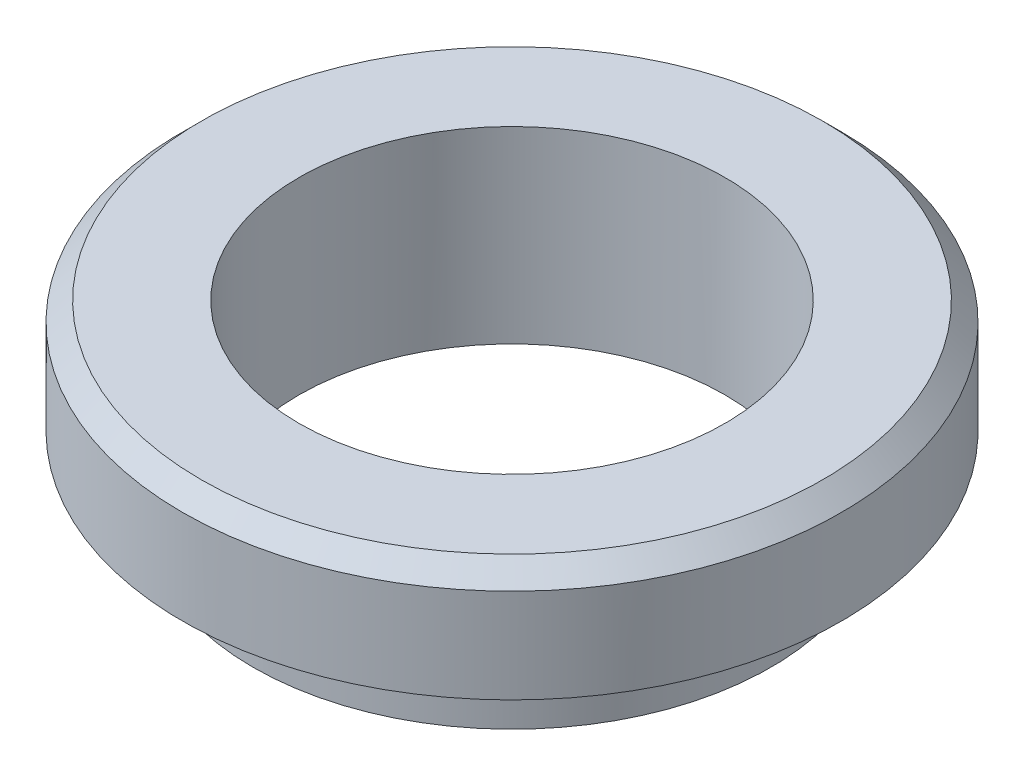
from build123d import *

# Parameters (mm, degrees)
G1_1_2_TAPPED_HOLE1_D     = 45.25
G1_1_2_TAPPED_HOLE1_DEPTH = 102.54
G1_1_2_TAPPED_HOLE1_TIP   = 13.594471505
CHAMFER1_SIZE             = 2


with BuildPart() as part:
    # Sketch1 → Revolve1 (revolve)
    with BuildSketch(Plane.XY, mode=Mode.PRIVATE) as revolve1_sk:
        Polygon((0, 0), (35, 0), (35, -12), (27.5, -12), (27.5, -20), (0, -20), align=None)
    revolve(revolve1_sk.sketch.rotate(Axis((0, -20, 0), (0, 1, 0)), 90), axis=Axis((0, -20, 0), (0, 1, 0)))

    # G1-1/2 Tapped Hole1
    with Locations(Plane(origin=(0, 0, 0), x_dir=(1, 0, 0), z_dir=(0, 1, 0))):
        with Locations((0, 0)):
            Hole(G1_1_2_TAPPED_HOLE1_D / 2, depth=G1_1_2_TAPPED_HOLE1_DEPTH)
            with Locations((0, 0, -(G1_1_2_TAPPED_HOLE1_DEPTH + G1_1_2_TAPPED_HOLE1_TIP / 2))):  # 118° drill point
                Cone(0, G1_1_2_TAPPED_HOLE1_D / 2, G1_1_2_TAPPED_HOLE1_TIP, mode=Mode.SUBTRACT)

    # Chamfer1
    chamfer1_edges = [part.edges().sort_by_distance(p)[0] for p in [
        (0, 0, 35),
    ]]
    chamfer(chamfer1_edges, length=CHAMFER1_SIZE)


solid = part.part
